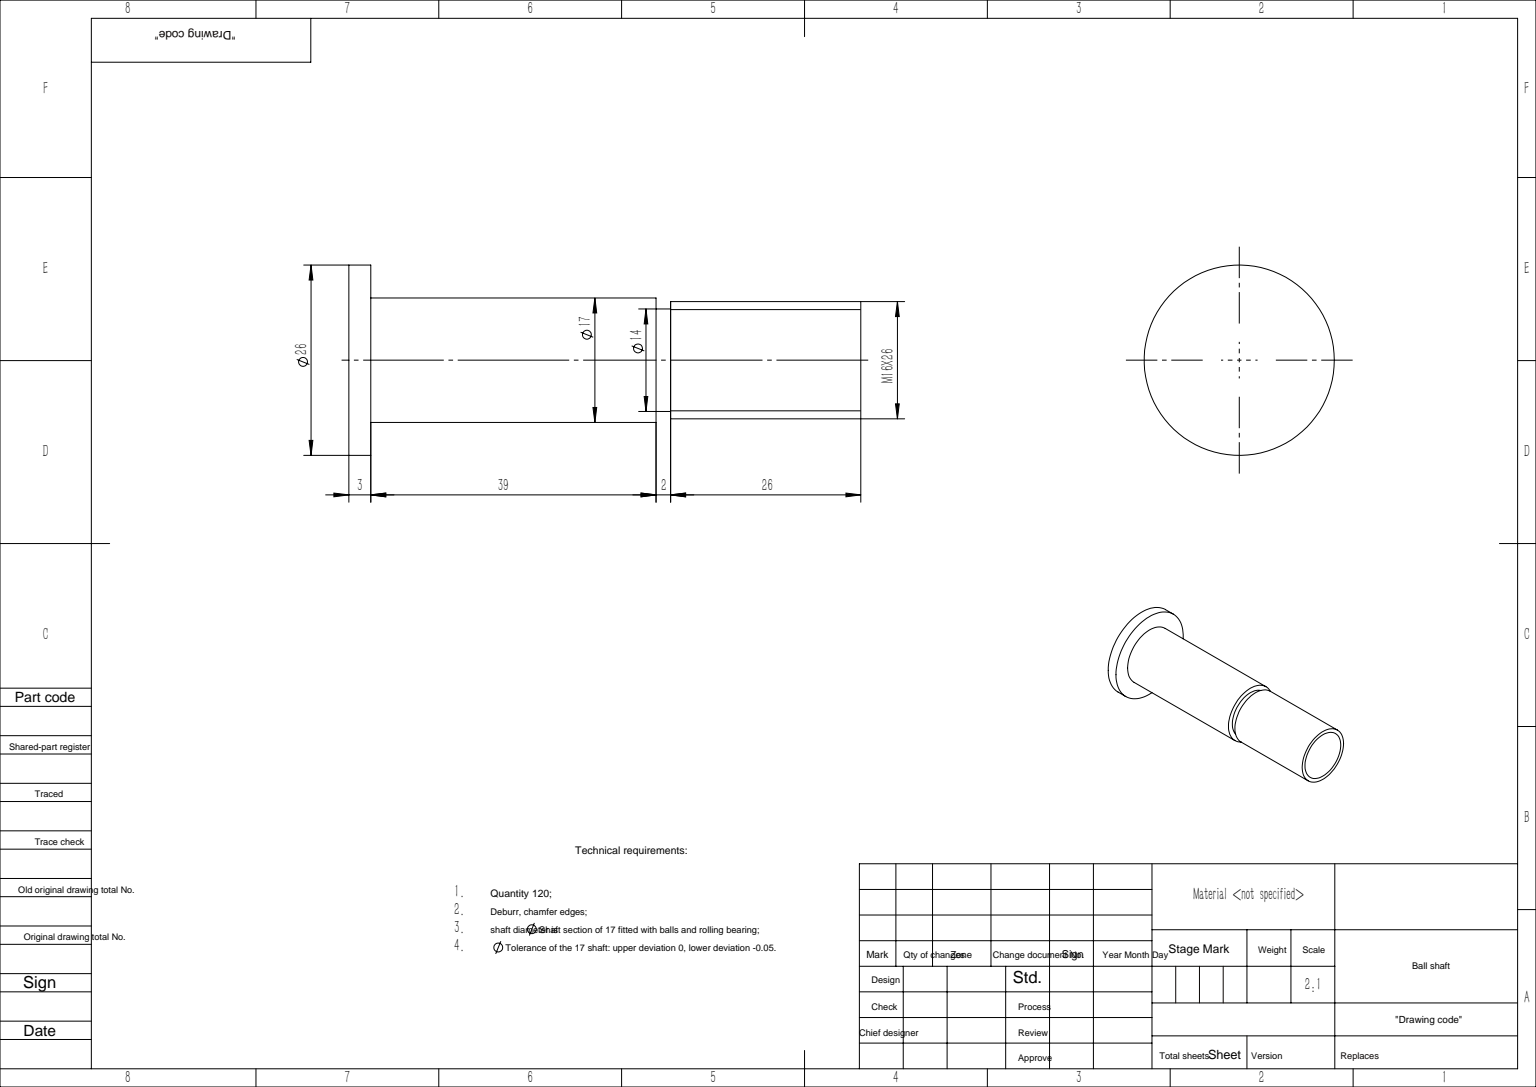
from build123d import *

# Parameters (mm, degrees)
SKETCH_2_R          = 8.5
SKETCH_2_R_2        = 8
CUT_EXTRUDE_1_DEPTH = 28
CUT_EXTRUDE_START   = 2
SKETCH_3_R          = 8
SKETCH_3_R_2        = 7
CUT_EXTRUDE_2_DEPTH = 2


with BuildPart() as part:
    # 草图1 → 旋转1 (revolve)
    with BuildSketch(Plane.XY, mode=Mode.PRIVATE) as revolve_1_sk:
        Polygon((0, 0), (0, 13), (3, 13), (3, 8.5), (70, 8.5), (70, 0), align=None)
    revolve(revolve_1_sk.sketch.rotate(Axis((0, 0, 0), (1, 0, 0)), 90), axis=Axis((0, 0, 0), (1, 0, 0)))

    # 草图2 → 切除-拉伸1 (cut)
    with BuildSketch(Plane(origin=(70, 0, 0), x_dir=(0, 0, -1), z_dir=(1, 0, 0))):
        with Locations(Location((0, 0, 0), (0, 0, 180))):
            Circle(SKETCH_2_R)
        Circle(SKETCH_2_R_2, mode=Mode.SUBTRACT)
    extrude(amount=-CUT_EXTRUDE_1_DEPTH, mode=Mode.SUBTRACT)

    # 草图3 → 切除-拉伸2 (cut)
    with BuildSketch(Plane(origin=(42, 0, 0), x_dir=(0, 0, -1), z_dir=(1, 0, 0)).offset(CUT_EXTRUDE_START)):
        Circle(SKETCH_3_R)
        Circle(SKETCH_3_R_2, mode=Mode.SUBTRACT)
    extrude(amount=-CUT_EXTRUDE_2_DEPTH, mode=Mode.SUBTRACT)


solid = part.part
